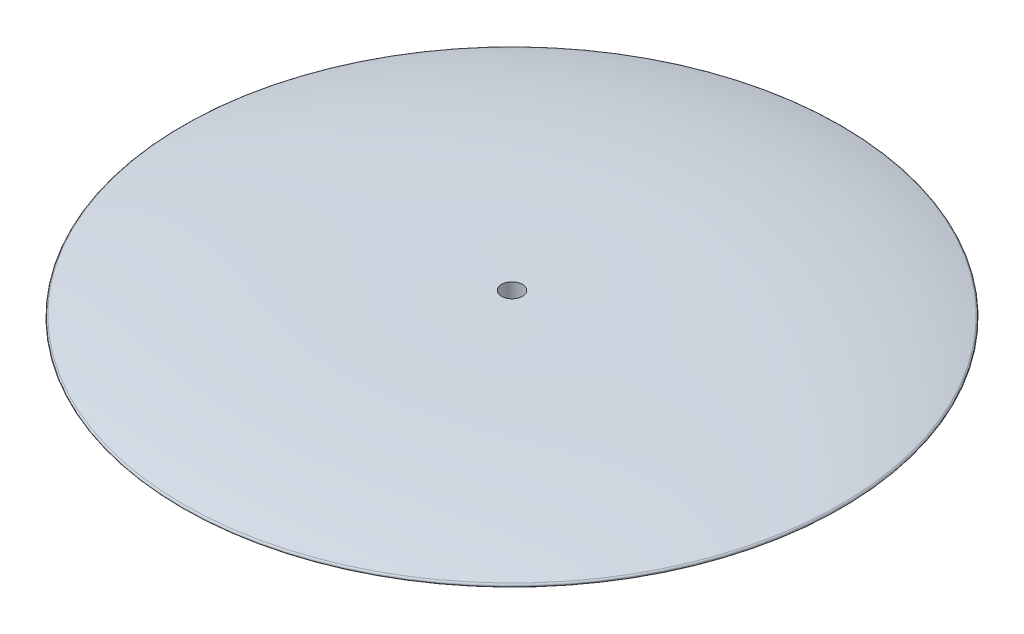
from build123d import *

# Parameters (mm, degrees)
FILLET_1_R          = 0.5
SKETCH_2_R          = 3
CUT_EXTRUDE_1_DEPTH = 23


with BuildPart() as part:
    # 草图1 → 旋转1 (revolve)
    with BuildSketch(Plane.XY):
        with BuildLine():
            Line((0, 0), (0, -5))
            add(Edge.make_bspline(
                [(-100, -7.814294025), (-72.076817605, -4.022924744), (-21.093053963, -5), (0, -5)],
                knots=[0, 0, 0, 0, 1, 1, 1, 1], degree=3))
            add(Edge.make_bspline(
                [(-100, -7.814294025), (-70.101614167, 2.125878409), (-22.774788705, 0), (0, 0)],
                knots=[0, 0, 0, 0, 1, 1, 1, 1], degree=3))
        make_face()
    revolve(axis=Axis((0, 0, 0), (0, -1, 0)))

    # 圆角1
    fillet_1_edges = [part.edges().sort_by_distance(p)[0] for p in [
        (100, -7.814294025, 0),
    ]]
    fillet(fillet_1_edges, radius=FILLET_1_R)

    # 草图2 → 切除-拉伸1 (cut, symmetric)
    with BuildSketch(Plane(origin=(0, 0, 0), x_dir=(1, 0, 0), z_dir=(0, 1, 0))):
        with Locations(Location((0, 0, 0), (0, 0, 270))):
            Circle(SKETCH_2_R)
    extrude(amount=CUT_EXTRUDE_1_DEPTH, both=True, mode=Mode.SUBTRACT)


solid = part.part
